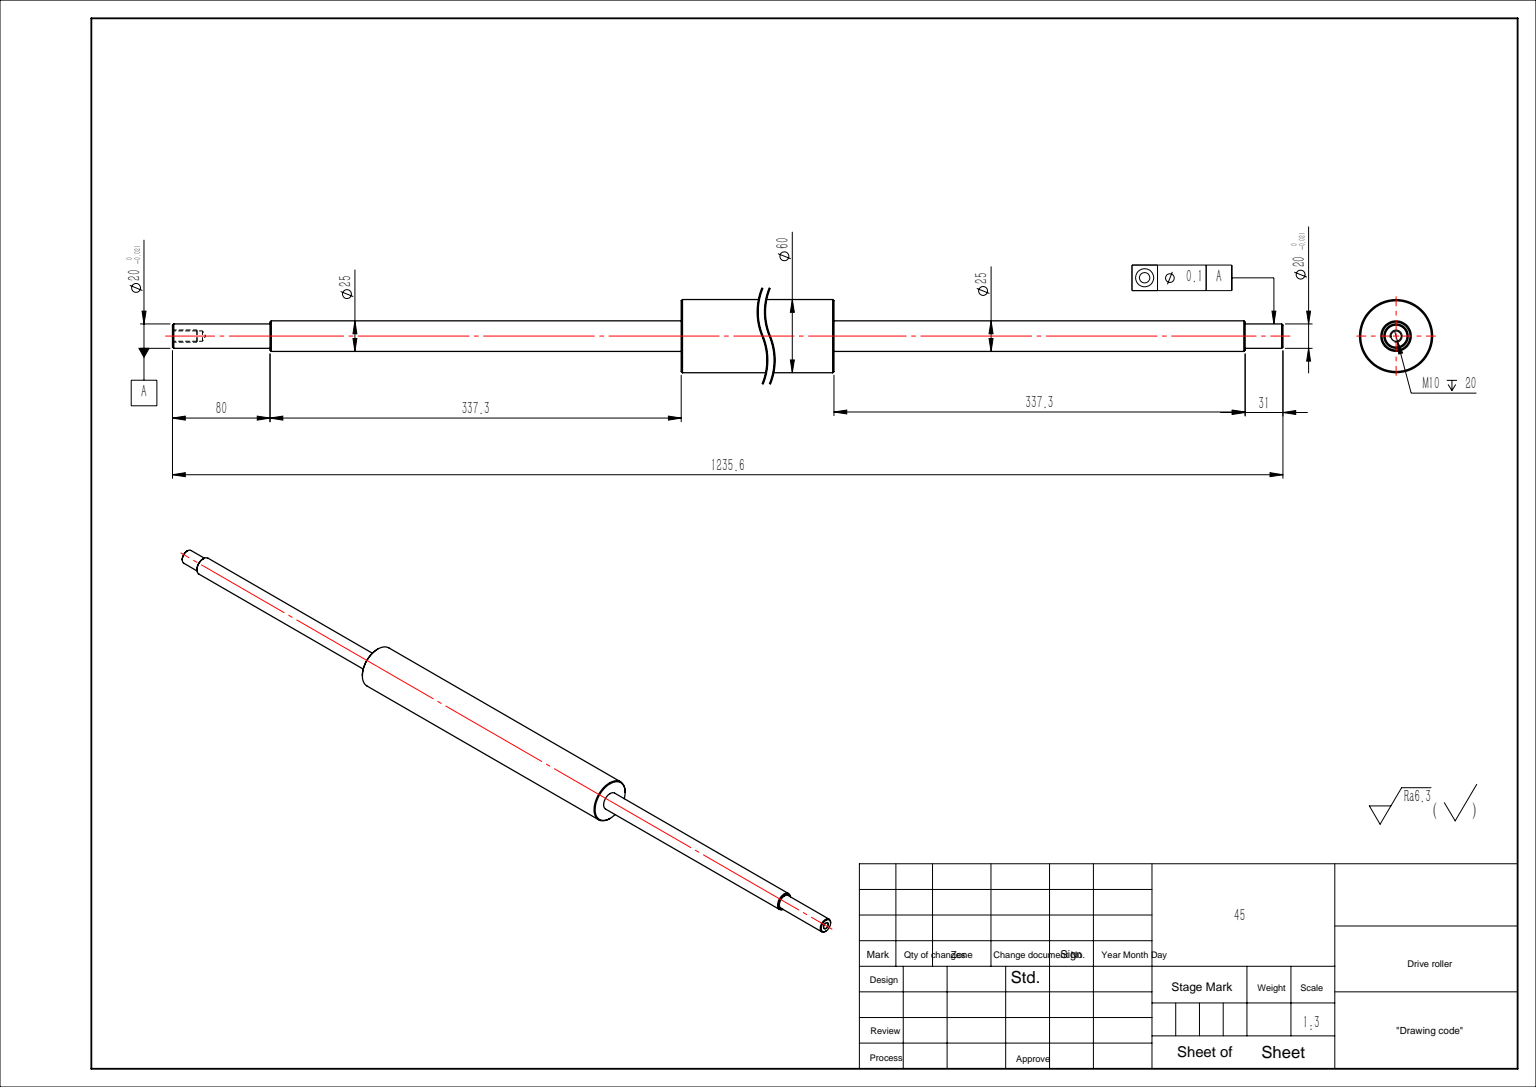
from build123d import *

# Parameters (mm, degrees)
CHAMFER_1_SIZE          = 1
HOLE_WIZARD_M10_1_D     = 8.5
HOLE_WIZARD_M10_1_DEPTH = 24.5
HOLE_WIZARD_M10_1_TIP   = 2.553657631


with BuildPart() as part:
    # 草图1 → 旋转1 (revolve)
    with BuildSketch(Plane.XY):
        Polygon((-593.3, 0), (-593.3, 10), (-562.3, 10), (-562.3, 12.5), (-225, 12.5), (-225, 30), (225, 30), (225, 12.5), (562.3, 12.5), (562.3, 10), (642.3, 10), (642.3, 0), align=None)
    revolve(axis=Axis((642.3, 0, 0), (-1, 0, 0)))

    # 倒角1
    chamfer_1_edges = [part.edges().sort_by_distance(p)[0] for p in [
        (225, -30, 0),
        (-225, -30, 0),
        (-562.3, -12.5, 0),
        (-593.3, -10, 0),
        (642.3, -10, 0),
        (562.3, -12.5, 0),
    ]]
    chamfer(chamfer_1_edges, length=CHAMFER_1_SIZE)

    # M10 螺纹孔1
    with Locations(Plane(origin=(642.3, 0, 0), x_dir=(0, 0, -1), z_dir=(1, 0, 0))):
        with Locations((0, 0)):
            Hole(HOLE_WIZARD_M10_1_D / 2, depth=HOLE_WIZARD_M10_1_DEPTH)
            with Locations((0, 0, -(HOLE_WIZARD_M10_1_DEPTH + HOLE_WIZARD_M10_1_TIP / 2))):  # 118° drill point
                Cone(0, HOLE_WIZARD_M10_1_D / 2, HOLE_WIZARD_M10_1_TIP, mode=Mode.SUBTRACT)


solid = part.part
